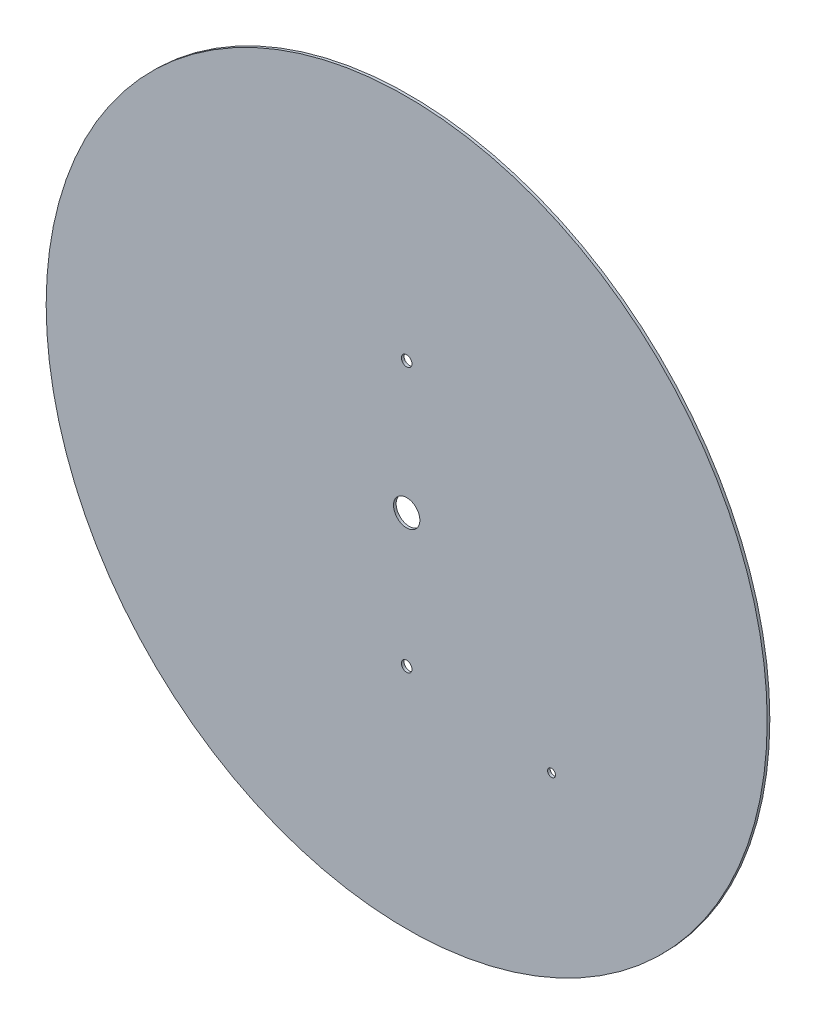
SolidWorks part; units mm, degrees
ref_plane "Front plane" through (0, 0, 0) normal (0, 0, 1) x (1, 0, 0)
ref_plane "Top plane" through (0, 0, 0) normal (0, 1, 0) x (1, 0, 0)
ref_plane "Right plane" through (0, 0, 0) normal (1, 0, 0) x (0, 0, -1)
sketch "Sketch 1" plane through (0, 0, 0) normal (0, 0, 1) x (1, 0, 0)
  circle A0 centre (0, 0) radius 68.5
  dimension "D1" = 137
extrude "Boss-Extrude 1" add sketch "Sketch 1" along normal blind 0.5
sketch "Sketch 2" plane through (0, 0, 0) normal (0, 0, -1) x (-1, 0, 0)
  circle A0 centre (0, 0) radius 2.5
  dimension "D1" = 5
extrude "Cut-Extrude 1" cut sketch "Sketch 2" against normal up to next
sketch "Sketch 3" plane through (0, 0, 0) normal (0, 0, -1) x (-1, 0, 0)
  circle A0 centre (0, 25) radius 1
  dimension "D1" = 2
  dimension "D2" = 25
extrude "Cut-Extrude 2" cut sketch "Sketch 3" against normal up to next
sketch "Sketch 4" plane through (0, 0, 0) normal (0, 0, -1) x (-1, 0, 0)
  line L0 (0, 0) -> (0, 68.5) construction
  line L1 (0, 0) -> (-47.1223, -49.7166) construction
  circle A0 centre (0, 0) radius 68.5 construction
  circle A1 centre (-27.5167, -29.0316) radius 0.75
  dimension "D2" = 1.5
  dimension "D1" = 136.535
  dimension "D3" = 40
extrude "Cut-Extrude 3" cut sketch "Sketch 4" against normal up to next
sketch "Sketch 5" plane through (0, 0, 0) normal (0, 0, -1) x (-1, 0, 0)
  line L0 (0, 0) -> (-48.4368, -48.4368) construction
  line L2 (-42.78, -42.0729) -> (-32.1734, -31.4663)
  line L3 (-42.78, -42.0729) -> (-42.0729, -42.78)
  line L4 (-42.0729, -42.78) -> (-31.4663, -32.1734)
  line L5 (-32.1734, -31.4663) -> (-31.4663, -32.1734)
  line L6 (-42.78, -42.0729) -> (-31.4663, -32.1734) construction
  line L7 (-42.0729, -42.78) -> (-32.1734, -31.4663) construction
  circle A0 centre (0, 0) radius 68.5 construction
  point P5 (-37.1231, -37.1231)
  dimension "D1" = 15
  dimension "D2" = 52.5
  dimension "D3" = 1
extrude "Boss-Extrude 2" add sketch "Sketch 5" along normal blind 0.5
pattern_circular "Circular pattern 1" count 9 over 270 about axis through (0, 0, 0) along (0, 0, 1) of "Boss-Extrude 2"
sketch "Sketch 6" plane through (0, 0, 0) normal (0, 0, -1) x (-1, 0, 0)
  line L0 (0, 0) -> (-48.4368, -48.4368) construction
  line L1 (0, 0) -> (-67.1838, -13.3637) construction
  line L2 (-44.2329, -8.2887) -> (-58.9447, -11.215) construction
  line L3 (0, 0) -> (-51.2043, -45.5013) construction
  line L5 (-45.1826, -39.4814) -> (-37.7075, -32.8389)
  line L6 (-45.1826, -39.4814) -> (-44.5184, -40.2289)
  line L7 (-44.5184, -40.2289) -> (-37.0433, -33.5864)
  line L8 (-37.7075, -32.8389) -> (-37.0433, -33.5864)
  line L9 (-45.1826, -39.4814) -> (-37.0433, -33.5864) construction
  line L10 (-44.5184, -40.2289) -> (-37.7075, -32.8389) construction
  circle A0 centre (0, 0) radius 68.5 construction
  point P8 (-41.113, -36.5339)
  dimension "D1" = 3.375
  dimension "D2" = 1
  dimension "D3" = 10
  dimension "D4" = 55
extrude "Boss-Extrude 3" add sketch "Sketch 6" along normal blind 0.5
pattern_circular "Circular pattern 2" count 79 over 263.25 about axis through (0, 0, 0) along (0, 0, 1) skipping 9, 19, 29, 39, 49, 59, 69 of "Boss-Extrude 3"
sketch "Sketch 7" plane through (0, 0, 0) normal (0, 0, -1) x (-1, 0, 0)
  line L0 (0, -3.8606) -> (0, 21.1394) construction
  circle A0 centre (0, -25.26) radius 1
  dimension "D2" = 2
  dimension "D1" = 25.26
extrude "Cut-Extrude 4" cut sketch "Sketch 7" against normal up to next
